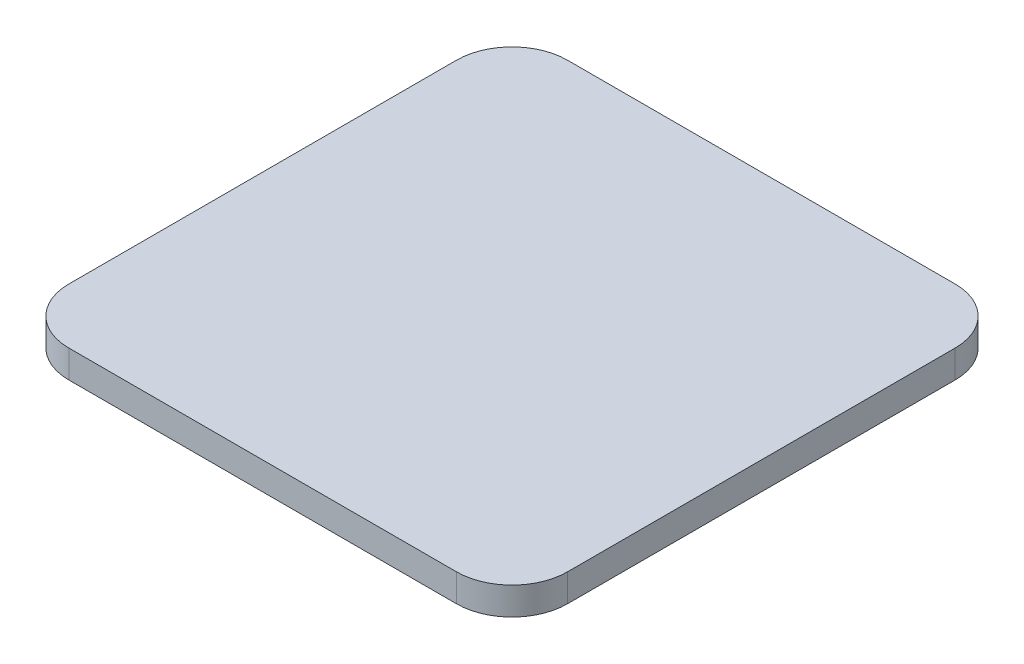
SolidWorks part; units mm, degrees
material "普通碳钢"
ref_plane "Front Plane" through (0, 0, 0) normal (0, 0, 1) x (1, 0, 0)
ref_plane "Top Plane" through (0, 0, 0) normal (0, 1, 0) x (1, 0, 0)
ref_plane "Right Plane" through (0, 0, 0) normal (1, 0, 0) x (0, 0, -1)
sketch "Sketch1" plane through (0, 0, 0) normal (0, 1, 0) x (1, 0, 0)
  line L5 (-18, 18) -> (18, 18)
  line L6 (-18, 18) -> (-18, -18)
  line L7 (-18, -18) -> (18, -18)
  line L8 (18, 18) -> (18, -18)
  line L9 (-18, 18) -> (18, -18) construction
  line L10 (-18, -18) -> (18, 18) construction
  point P0 (0, 0)
  dimension "D1" = 36
  dimension "D2" = 36
extrude "Boss-Extrude1" add sketch "Sketch1" along normal mid plane 2
fillet "Fillet1" radius 4 4 edges at (-18, 0, 18) (18, 0, 18) (18, 0, -18) (-18, 0, -18)
